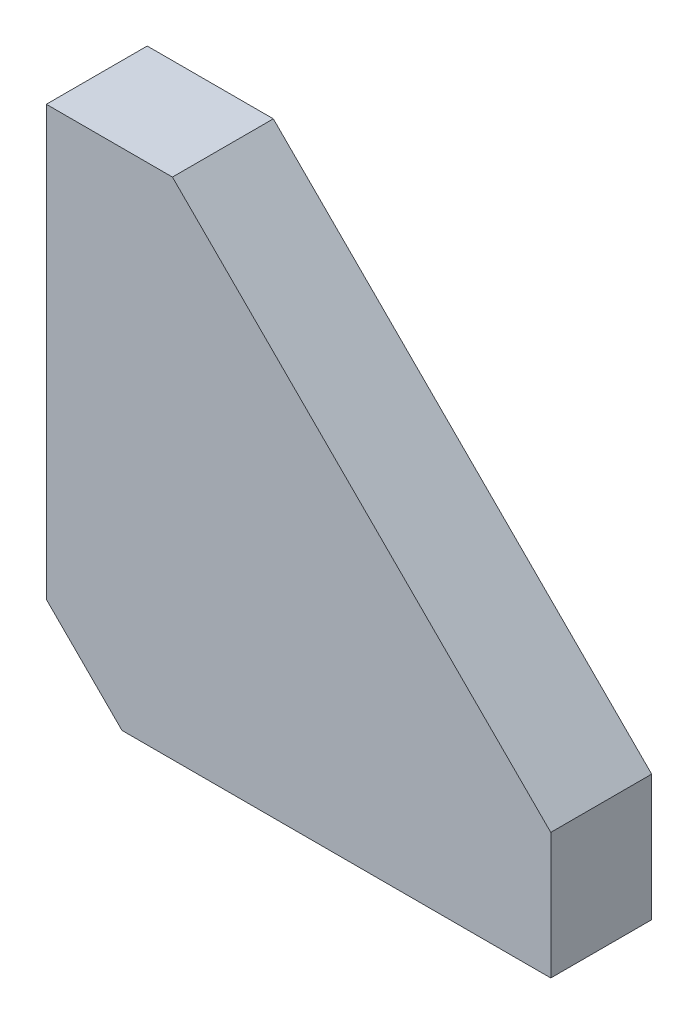
SolidWorks part; units mm, degrees
material "Q235"
ref_plane "Front Plane" through (0, 0, 0) normal (0, 0, 1) x (1, 0, 0)
ref_plane "Top Plane" through (0, 0, 0) normal (0, 1, 0) x (1, 0, 0)
ref_plane "Right Plane" through (0, 0, 0) normal (1, 0, 0) x (0, 0, -1)
sketch "Sketch1" plane through (0, 0, 0) normal (0, 0, 1) x (1, 0, 0)
  line L0 (0, 0) -> (100, 0)
  line L1 (100, 0) -> (100, 25)
  line L2 (100, 25) -> (25, 100)
  line L3 (25, 100) -> (0, 100)
  line L4 (0, 100) -> (0, 0)
  dimension "D1" = 100
  dimension "D2" = 100
  dimension "D3" = 25
  dimension "D4" = 25
extrude "Boss-Extrude1" add sketch "Sketch1" along normal blind 20
chamfer "Chamfer1" distance 15 angle 45 1 edges at (0, 0, 10)
